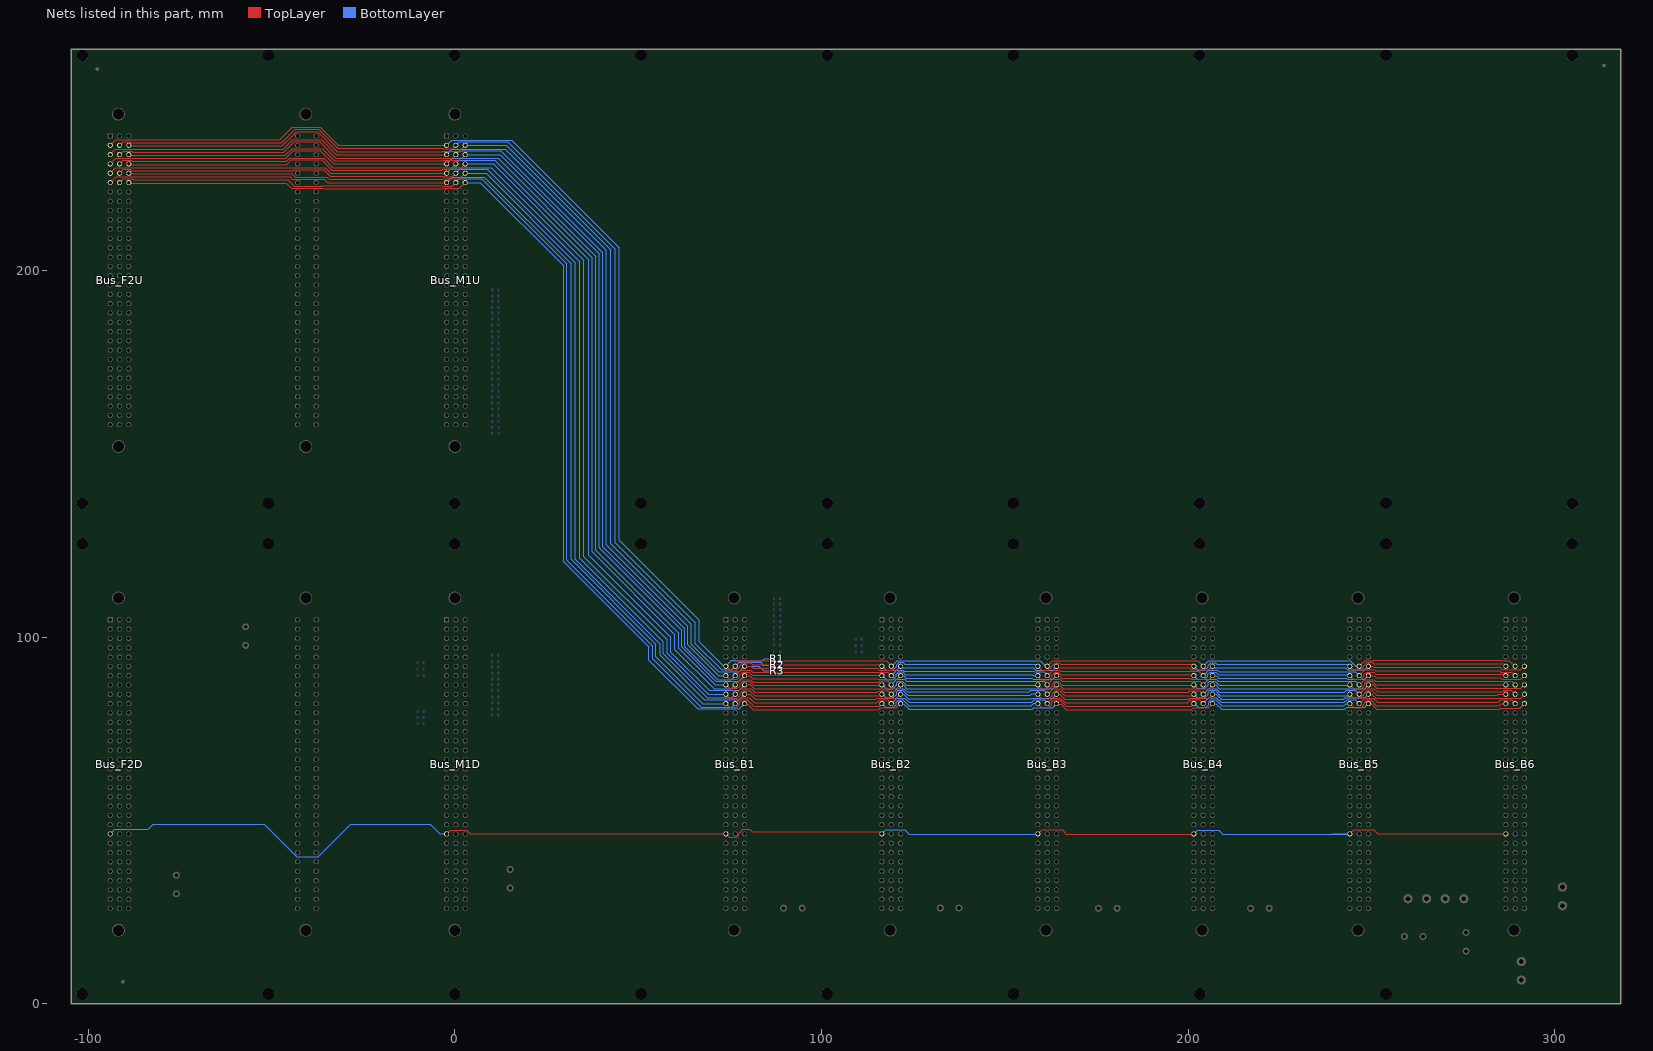
[diagram p0: the nets of this part, all layers, seen from the top]
# Altium PCB MISC67337.PcbDoc (part 4 of 7)
Units mm, origin at the board's own origin, x right, y up, seen from the top; angles counter-clockwise.
Board outline 422.71 x 260.35 mm, 4 copper layers (TopLayer, InternalPlane1, InternalPlane2, BottomLayer); 82 components, 143 nets, 1295 pads, 42 vias.

## Via types
v1: diameter 0.61, hole 0.305, TopLayer to BottomLayer, 42 vias

## Nets (pads, with @x,y where several pads share a name; then routed paths per layer and width w, separated by ;. In a path a pad name is that pad's centre, name@x,y a point inside that pad or via, vN(x,y) a via of type N, cw(c..) or ccw(c..) an arc to the next point about the centre after c; other vN are vias at no path point) (continued)
B_DSP1_XD15: Bus_B1.A24 Bus_B2.A24 Bus_B3.A24 Bus_B4.A24 Bus_B5.A24 Bus_B6.A24 Bus_F2D.A24 Bus_M1D.A24 | length 404.9
  TopLayer w0.254: Bus_M1D.A24@-2.24,46.274 -1.262,47.252 3.245,47.252 4.204,46.293 Bus_B1.A24@73.955,46.293 74.933,45.315 76.9,45.315 77.473,45.888 77.473,46.358 78.613,47.498 80.493,47.498 81.102,46.888 115.91,46.888 Bus_B2.A24@116.505,46.293 ; Bus_B3.A24@159.05,46.166 160.255,47.371 165.633,47.371 166.839,46.165 Bus_B4.A24@201.406,46.165 ; Bus_B4.A24@201.406,46.355 Bus_B4.A24@201.595,46.166 ; Bus_B5.A24@244.14,46.293 245.218,47.371 250.723,47.371 251.801,46.293 Bus_B6.A24@286.685,46.293
  BottomLayer w0.254: Bus_F2D.A24@-93.97,46.274 -92.72,47.523 -83.566,47.523 -82.22,48.87 -52.019,48.87 -43.155,40.005 -37.262,40.005 -28.346,48.92 -6.706,48.92 -4.059,46.274 Bus_M1D.A24@-2.24,46.274 ; Bus_B2.A24@116.505,46.293 117.583,47.371 122.784,47.371 123.896,46.259 151.867,46.259 ; 153.389,46.259 151.867,46.259 ; Bus_B3.A24@159.05,46.293 159.016,46.259 151.867,46.259 ; Bus_B4.A24@201.595,46.293 202.622,47.32 208.407,47.32 209.501,46.227 236.652,46.227 ; 238.352,46.227 236.652,46.227 ; 239.349,46.274 Bus_B5.A24@244.121,46.274 ; Bus_B5.A24@244.14,46.293 Bus_B5.A24@244.121,46.274 ; 236.652,46.227 244.074,46.227 Bus_B5.A24@244.121,46.274
B_DSP2_C\S\: Bus_B1.A6 Bus_B2.A6 Bus_B3.A6 Bus_B4.A6 Bus_B5.A6 Bus_B6.A6 Bus_F2U.A2 Bus_M1U.A2 R1.2 | length 531.8
  TopLayer w0.254: Bus_F2U.A2@-93.97,234.113 -92.473,235.61 -47.701,235.61 -44.298,239.014 -36.728,239.014 -31.828,234.113 Bus_M1U.A2@-2.24,234.113 ; Bus_B1.A6@73.96,92.14 75.295,90.805 76.67,90.805 77.724,91.859 77.724,92.207 78.508,92.991 80.77,92.991 81.31,92.451 109.093,92.451 ; 115.654,92.451 109.093,92.451 ; Bus_B2.A6@116.505,92.013 116.067,92.451 109.093,92.451 ; Bus_B3.A6@159.05,92.013 160.131,90.932 161.925,90.932 162.814,91.821 162.814,92.08 163.725,92.991 164.76,92.991 165.227,92.524 198.374,92.524 ; 200.617,92.524 198.374,92.524 ; Bus_B4.A6@201.595,92.013 201.084,92.524 198.374,92.524 ; Bus_B5.A6@244.14,92.013 245.118,91.035 247.245,91.035 247.904,91.694 247.904,92.08 248.89,93.066 250.19,93.066 250.609,92.646 283.337,92.646 ; 285.707,92.646 283.337,92.646 ; Bus_B6.A6@286.685,92.013 286.052,92.646 283.337,92.646
  BottomLayer w0.254: Bus_M1U.A2@-2.24,234.113 -0.856,235.498 15.505,235.498 44.831,206.172 44.831,126.365 66.675,104.521 66.675,98.679 73.341,92.013 Bus_B1.A6@73.955,92.013 75.538,93.596 76.07,93.596 76.09,93.575 83.796,93.575 84.353,94.132 R1.2@87.097,94.132 ; Bus_B2.A6@116.632,92.075 117.713,90.994 119.507,90.994 120.523,92.01 120.523,92.391 121.185,93.053 122.215,93.053 122.682,92.586 157.505,92.586 ; 158.199,92.586 157.505,92.586 ; Bus_B3.A6@159.05,92.013 158.477,92.586 157.505,92.586 ; Bus_B4.A6@201.595,92.013 202.676,90.932 204.47,90.932 205.486,91.948 205.486,92.329 206.148,92.991 207.411,92.991 207.874,92.528 241.783,92.528 ; 243.162,92.528 241.783,92.528 ; Bus_B5.A6@244.14,92.013 243.625,92.528 241.783,92.528
B_DSP2_X\R\D\: Bus_B1.B6 Bus_B2.B6 Bus_B3.B6 Bus_B4.B6 Bus_B5.B6 Bus_B6.B6 Bus_F2U.B2 Bus_M1U.B2 R2.1 | length 514.3
  TopLayer w0.254: Bus_F2U.B2@-91.43,234.113 -90.452,235.091 -88.485,235.091 -88.161,234.767 -50.317,234.767 ; -49.555,234.767 -50.317,234.767 ; Bus_M1U.B2@0.3,234.113 -0.678,233.136 -3.316,233.136 -3.448,233.267 -31.946,233.267 -37.135,238.455 -43.536,238.455 -47.223,234.767 -50.317,234.767 ; Bus_B1.B6@76.5,92.14 77.908,93.548 117.637,93.548 Bus_B2.B6@119.045,92.14 ; Bus_B3.B6@161.59,92.013 163.049,93.472 202.676,93.472 Bus_B4.B6@204.135,92.013 ; Bus_B5.B6@246.68,92.013 248.242,93.575 250.674,93.575 250.698,93.599 285.496,93.599 285.52,93.575 287.663,93.575 Bus_B6.B6@289.225,92.013
  BottomLayer w0.254: Bus_M1U.B2@0.3,234.113 1.278,235.091 14.489,235.091 43.815,205.765 43.815,125.73 65.659,103.886 65.659,98.171 72.795,91.035 75.517,91.035 Bus_B1.B6@76.495,92.013 77.573,93.091 83.439,93.091 84.201,92.329 87.046,92.329 R2.1@87.097,92.38 ; Bus_B2.B6@119.172,92.075 120.631,93.534 159.704,93.534 161.163,92.075 Bus_B3.B6@161.717,92.075 ; Bus_B4.B6@204.135,92.013 205.594,93.472 244.221,93.472 245.68,92.013 Bus_B5.B6@246.68,92.013
B_DSP2_X\W\E\: Bus_B1.C6 Bus_B2.C6 Bus_B3.C6 Bus_B4.C6 Bus_B5.C6 Bus_B6.C6 Bus_F2U.C2 Bus_M1U.C2 R3.2 | length 513.4
  TopLayer w0.254: Bus_F2U.C2@-88.89,233.924 -47.025,233.924 -43.921,237.028 ; -43.921,237.032 -43.21,237.744 -37.363,237.744 -32.039,232.42 -3.368,232.42 -3.237,232.551 1.278,232.551 Bus_M1U.C2@2.84,234.113 1.391,232.664 ; Bus_B1.C6@79.035,92.013 80.859,92.013 81.367,91.505 112.827,91.505 ; 113.473,91.505 112.827,91.505 ; Bus_B2.C6@121.585,92.14 120.377,90.932 115.849,90.932 115.276,91.505 112.827,91.505 ; Bus_B3.C6@164.13,91.575 198.145,91.575 ; 198.563,91.575 198.145,91.575 ; Bus_B4.C6@206.675,92.013 205.697,91.035 200.887,91.035 200.347,91.575 198.145,91.575 ; Bus_B5.C6@249.22,92.013 249.282,92.075 250.317,92.075 250.698,91.694 283.718,91.694 ; 284.796,91.694 283.718,91.694 ; Bus_B6.C6@291.765,92.013 290.787,91.035 285.774,91.035 285.115,91.694 283.718,91.694
  BottomLayer w0.254: Bus_M1U.C2@2.84,234.113 14.019,234.113 42.545,205.588 42.545,125.476 64.516,103.505 64.516,98.044 72.009,90.551 77.573,90.551 Bus_B1.C6@79.035,92.013 82.969,92.013 84.228,90.754 R3.2@87.097,90.754 ; Bus_B2.C6@121.712,91.638 156.642,91.638 ; 157.353,91.638 156.642,91.638 ; Bus_B3.C6@164.257,92.075 163.114,90.932 158.496,90.932 157.79,91.638 156.642,91.638 ; Bus_B4.C6@206.675,91.584 241.859,91.584 ; 242.632,91.584 241.859,91.584 ; Bus_B5.C6@249.22,92.013 248.242,91.035 243.61,91.035 243.061,91.584 241.859,91.584
B_DSP2_XA0: Bus_B1.A7 Bus_B2.A7 Bus_B3.A7 Bus_B4.A7 Bus_B5.A7 Bus_B6.A7 Bus_F2U.A3 Bus_M1U.A3 | length 507.2
  TopLayer w0.254: Bus_F2U.A3@-93.97,231.573 -93.97,231.658 -92.583,233.045 ; -92.583,233.081 -46.725,233.081 -44.221,235.585 -36.297,235.585 -32.285,231.573 Bus_M1U.A3@-2.24,231.573 ; Bus_B1.A7@73.96,89.473 74.938,88.495 77.065,88.495 77.724,89.154 77.724,89.667 78.508,90.451 80.313,90.451 81.151,89.613 112.141,89.613 ; 112.649,89.613 112.141,89.613 ; Bus_B2.A7@116.505,89.473 116.365,89.613 112.141,89.613 ; Bus_B3.A7@159.05,89.346 160.028,88.368 162.155,88.368 162.814,89.027 162.814,89.54 163.725,90.451 164.667,90.451 165.439,89.679 197.307,89.679 ; 197.739,89.679 197.307,89.679 ; Bus_B4.A7@201.595,89.346 201.468,89.473 Bus_B4.A7@201.595,89.473 201.389,89.679 197.307,89.679 ; Bus_B5.A7@244.14,89.473 245.118,88.495 247.245,88.495 248.031,89.281 248.031,89.789 248.693,90.451 250.671,90.451 251.333,89.789 Bus_B6.A7@286.685,89.789
  BottomLayer w0.254: Bus_M1U.A3@-2.24,231.573 -0.768,233.045 13.716,233.045 41.275,205.486 41.275,125.095 63.5,102.87 63.5,97.917 71.944,89.473 Bus_B1.A7@73.955,89.473 ; Bus_B2.A7@116.632,89.535 117.775,88.392 119.445,88.392 120.396,89.343 120.396,89.851 121.058,90.513 122.136,90.513 122.907,89.742 155.981,89.742 ; 156.818,89.742 155.981,89.742 ; Bus_B3.A7@159.05,89.473 157.858,89.473 157.589,89.742 155.981,89.742 ; Bus_B3.A7@159.05,89.535 Bus_B3.A7@159.177,89.535 ; Bus_B4.A7@201.595,89.473 202.573,88.495 204.573,88.495 205.359,89.281 205.359,89.789 206.021,90.451 207.618,90.451 208.373,89.696 240.462,89.696 ; 241.781,89.696 240.462,89.696 ; Bus_B5.A7@244.14,89.473 243.917,89.696 240.462,89.696
B_DSP2_XA1: Bus_B1.B7 Bus_B2.B7 Bus_B3.B7 Bus_B4.B7 Bus_B5.B7 Bus_B6.B7 Bus_F2U.B3 Bus_M1U.B3 | length 503.5
  TopLayer w0.254: Bus_F2U.B3@-91.43,231.573 -90.452,232.551 -88.121,232.551 -87.808,232.238 -46.603,232.238 -43.764,235.077 -41.758,235.077 ; -41.631,235.077 -41.758,235.077 ; Bus_M1U.B3@0.3,231.573 -0.678,230.596 -32.399,230.596 -36.881,235.077 -41.758,235.077 ; Bus_B1.B7@76.495,89.473 78.006,90.984 80.72,90.984 81.253,90.451 118.067,90.451 Bus_B2.B7@119.045,89.473 ; Bus_B1.B7@76.5,89.473 77.626,90.599 ; Bus_B3.B7@161.59,89.346 163.176,90.932 164.922,90.932 165.227,90.627 202.981,90.627 Bus_B4.B7@204.135,89.473 ; Bus_B4.B7@204.071,89.41 Bus_B4.B7@204.135,89.346 ; Bus_B5.B7@246.68,89.473 248.241,91.034 250.8,91.034 251.092,90.742 285.002,90.742 285.293,90.451 288.247,90.451 Bus_B6.B7@289.225,89.473
  BottomLayer w0.254: Bus_M1U.B3@0.3,231.573 1.365,232.639 12.548,232.639 40.386,204.8 40.386,124.587 62.738,102.235 62.738,97.409 71.755,88.392 75.414,88.392 Bus_B1.B7@76.495,89.473 ; Bus_B2.B7@119.172,89.535 120.62,90.983 122.338,90.983 122.631,90.69 122.682,90.69 157.251,90.69 ; 157.618,90.69 157.251,90.69 ; Bus_B3.B7@161.717,89.535 160.726,90.526 158.075,90.526 157.911,90.69 157.251,90.69 ; Bus_B4.B7@204.135,89.473 205.645,90.983 207.95,90.983 208.458,90.475 245.678,90.475 Bus_B5.B7@246.68,89.473
B_DSP2_XA2: Bus_B1.C7 Bus_B2.C7 Bus_B3.C7 Bus_B4.C7 Bus_B5.C7 Bus_B6.C7 Bus_F2U.C3 Bus_M1U.C3 | length 499.4
  TopLayer w0.254: Bus_F2U.C3@-88.89,231.395 -46.176,231.395 -44.372,233.199 -36.12,233.199 -32.801,229.88 -3.317,229.88 -3.186,230.011 1.278,230.011 Bus_M1U.C3@2.84,231.573 ; Bus_B1.C7@79.035,89.473 80.428,89.473 81.233,88.668 115.372,88.668 115.545,88.495 ; 115.519,88.495 115.545,88.495 ; Bus_B2.C7@121.585,89.473 120.607,88.495 115.545,88.495 ; Bus_B3.C7@164.13,89.473 164.832,89.473 165.575,88.73 197.206,88.73 ; 197.485,88.73 197.206,88.73 ; Bus_B4.C7@206.675,89.346 205.824,88.495 203.73,88.495 203.728,88.494 202.002,88.494 202,88.495 200.863,88.495 200.628,88.73 197.206,88.73 ; Bus_B5.C7@249.22,89.473 250.735,89.473 251.371,88.837 285.356,88.837 285.698,88.495 287.09,88.495 287.114,88.519 288.796,88.519 288.82,88.495 290.787,88.495 Bus_B6.C7@291.765,89.473
  BottomLayer w0.254: Bus_M1U.C3@2.84,231.573 12.343,231.573 39.37,204.546 39.37,124.333 61.849,101.854 61.849,97.282 71.22,87.911 77.473,87.911 Bus_B1.C7@79.035,89.473 ; Bus_B2.C7@121.585,89.473 122.414,89.473 123.093,88.794 156.032,88.794 ; 156.653,88.794 156.032,88.794 ; Bus_B3.C7@164.257,89.535 163.165,88.443 157.745,88.443 157.394,88.794 156.032,88.794 ; Bus_B4.C7@206.675,89.473 207.682,89.473 208.402,88.752 240.665,88.752 ; 241.616,88.752 240.665,88.752 ; Bus_B5.C7@249.22,89.473 248.242,88.495 243.586,88.495 243.329,88.752 240.665,88.752
B_DSP2_XA3: Bus_B1.A8 Bus_B2.A8 Bus_B3.A8 Bus_B4.A8 Bus_B5.A8 Bus_B6.A8 Bus_F2U.A4 Bus_M1U.A4 | length 507.8
  TopLayer w0.254: Bus_F2U.A4@-93.97,229.033 -92.451,230.552 -46.105,230.552 -43.993,232.664 -36.703,232.664 -33.072,229.033 Bus_M1U.A4@-2.24,229.033 ; Bus_B1.A8@73.96,86.933 74.938,85.955 77.065,85.955 77.851,86.741 77.851,87.254 78.508,87.911 80.313,87.911 81.449,86.776 Bus_B2.A8@116.505,86.776 ; Bus_B3.A8@159.05,86.806 160.028,85.828 162.155,85.828 163.093,86.766 163.093,87.279 163.725,87.911 164.667,87.911 165.744,86.834 Bus_B4.A8@201.595,86.834 ; Bus_B5.A8@244.14,86.933 245.221,85.852 247.269,85.852 248.242,86.825 248.242,87.338 248.815,87.911 250.29,87.911 251.269,86.932 286.684,86.932 Bus_B6.A8@286.685,86.933
  BottomLayer w0.254: Bus_M1U.A4@-2.24,229.033 -0.678,230.596 11.797,230.596 38.481,203.911 38.481,123.698 61.087,101.092 61.087,96.901 71.055,86.933 Bus_B1.A8@73.955,86.933 ; Bus_B2.A8@116.632,86.995 117.902,85.725 119.318,85.725 120.523,86.93 120.523,87.565 120.931,87.973 122.034,87.973 123.11,86.898 154.254,86.898 ; 155.929,86.898 154.254,86.898 ; Bus_B3.A8@159.05,86.933 159.015,86.898 154.254,86.898 ; Bus_B4.A8@201.595,86.933 202.573,85.955 204.573,85.955 205.486,86.868 205.486,87.503 205.894,87.911 207.415,87.911 208.461,86.864 238.201,86.864 ; 240.892,86.864 238.201,86.864 ; Bus_B5.A8@244.14,86.933 244.071,86.864 238.201,86.864
B_DSP2_XA4: Bus_B1.B8 Bus_B2.B8 Bus_B3.B8 Bus_B4.B8 Bus_B5.B8 Bus_B6.B8 Bus_F2U.B4 Bus_M1U.B4 | length 500.6
  TopLayer w0.254: Bus_F2U.B4@-91.43,229.033 -90.452,230.011 -88.288,230.011 -87.986,229.709 -45.906,229.709 -44.983,230.632 -35.789,230.632 -33.212,228.056 -0.678,228.056 Bus_M1U.B4@0.3,229.033 ; Bus_B1.B8@76.5,86.933 77.968,88.402 80.559,88.402 81.239,87.722 111.328,87.722 ; 112.258,87.722 111.328,87.722 ; Bus_B2.B8@119.045,86.933 117.94,88.038 115.926,88.038 115.609,87.722 111.328,87.722 ; Bus_B3.B8@161.59,86.806 Bus_B3.B8@161.653,86.87 ; Bus_B3.B8@161.59,86.933 163.074,88.417 165.141,88.417 165.648,87.911 203.157,87.911 Bus_B4.B8@204.135,86.933 ; Bus_B4.B8@204.071,86.87 Bus_B4.B8@204.135,86.806 ; Bus_B5.B8@246.68,86.933 248.139,88.392 250.698,88.392 251.181,87.909 282.473,87.909 282.475,87.911 288.247,87.911 Bus_B6.B8@289.225,86.933
  BottomLayer w0.254: Bus_M1U.B4@0.3,229.033 1.278,230.011 3.245,230.011 3.259,229.997 10.947,229.997 37.465,203.479 37.465,123.19 60.071,100.584 60.071,96.52 70.739,85.852 75.414,85.852 Bus_B1.B8@76.495,86.933 ; Bus_B2.B8@119.045,86.933 120.529,88.417 122.695,88.417 123.139,87.973 160.739,87.973 Bus_B3.B8@161.717,86.995 ; Bus_B4.B8@204.135,86.933 205.619,88.417 207.696,88.417 208.202,87.911 245.702,87.911 Bus_B5.B8@246.68,86.933
B_DSP2_XA5: Bus_B1.C8 Bus_B2.C8 Bus_B3.C8 Bus_B4.C8 Bus_B5.C8 Bus_B6.C8 Bus_F2U.C4 Bus_M1U.C4 | length 501.5
  TopLayer w0.254: Bus_F2U.C4@-88.89,228.866 -45.835,228.866 -44.577,230.124 -36.271,230.124 -33.487,227.34 -3.394,227.34 -3.175,227.559 1.365,227.559 Bus_M1U.C4@2.84,229.033 ; Bus_B1.C8@79.035,86.933 80.529,86.933 81.632,85.83 114.3,85.83 ; 115.189,85.83 114.3,85.83 ; Bus_B2.C8@121.585,86.933 120.482,85.83 114.3,85.83 ; Bus_B3.C8@164.13,86.806 165.035,86.806 165.964,85.877 ; 165.964,85.885 205.746,85.885 ; 205.746,85.877 Bus_B4.C8@206.675,86.806 ; Bus_B5.C8@249.22,86.933 250.455,86.933 251.433,85.955 290.787,85.955 Bus_B6.C8@291.765,86.933
  BottomLayer w0.254: Bus_M1U.C4@2.84,229.033 10.438,229.033 36.576,202.895 36.576,122.301 58.928,99.949 58.928,95.885 69.367,85.446 77.548,85.446 Bus_B1.C8@79.035,86.933 ; Bus_B2.C8@121.585,86.933 122.338,86.933 123.321,85.949 153.924,85.949 ; Bus_B2.C8@121.712,86.995 Bus_B2.C8@122.028,87.311 ; 155.067,85.949 153.924,85.949 ; Bus_B3.C8@164.13,86.933 163.146,85.949 153.924,85.949 ; Bus_B3.C8@164.163,86.901 Bus_B3.C8@164.257,86.995 ; Bus_B4.C8@206.991,87.249 Bus_B4.C8@206.675,86.933 207.529,86.933 208.542,85.921 238.455,85.921 ; 240.03,85.921 238.455,85.921 ; Bus_B5.C8@249.22,86.933 248.208,85.921 238.455,85.921
B_DSP2_XA6: Bus_B1.A9 Bus_B2.A9 Bus_B3.A9 Bus_B4.A9 Bus_B5.A9 Bus_B6.A9 Bus_F2U.A5 Bus_M1U.A5 | length 506
  TopLayer w0.254: Bus_F2U.A5@-93.97,226.493 -92.498,227.965 ; -92.498,228.023 -35.288,228.023 -33.758,226.493 Bus_M1U.A5@-2.24,226.493 ; Bus_B1.A9@73.96,84.393 75.041,83.312 77.089,83.312 77.851,84.074 77.851,84.714 78.532,85.395 78.918,85.395 ; 79.654,85.395 78.918,85.395 ; Bus_B2.A9@116.505,84.393 116.05,83.938 81.899,83.938 80.442,85.395 78.918,85.395 ; Bus_B3.A9@159.05,84.266 160.131,83.185 162.179,83.185 162.941,83.947 162.941,84.587 163.725,85.371 164.997,85.371 166.379,83.988 201.19,83.988 Bus_B4.A9@201.531,84.33 ; Bus_B4.A9@201.152,84.709 Bus_B4.A9@201.531,84.33 ; Bus_B4.A9@201.595,84.266 Bus_B4.A9@201.531,84.33 ; Bus_B4.A9@201.595,84.393 Bus_B4.A9@201.531,84.33 ; Bus_B5.A9@244.14,84.393 245.118,83.415 247.118,83.415 248.242,84.539 248.242,84.798 248.815,85.371 250.239,85.371 251.536,84.074 253.111,84.074 ; 252.73,84.074 253.111,84.074 ; Bus_B6.A9@286.685,84.393 284.621,84.393 284.48,84.252 284.48,84.201 284.353,84.074 253.111,84.074
  BottomLayer w0.254: Bus_M1U.A5@-2.24,226.493 -0.768,227.965 10.008,227.965 35.179,202.794 35.179,121.92 57.912,99.187 57.912,95.631 69.15,84.393 Bus_B1.A9@73.955,84.393 ; Bus_B2.A9@116.632,84.455 117.672,83.415 119.515,83.415 120.523,84.423 120.523,85.025 121.031,85.533 122.137,85.533 123.617,84.053 124.409,84.053 124.435,84.079 ; 124.435,84.053 157.028,84.053 157.429,84.455 Bus_B3.A9@158.988,84.455 ; Bus_B3.A9@159.05,84.393 Bus_B3.A9@158.988,84.455 ; Bus_B3.A9@159.177,84.455 Bus_B3.A9@158.988,84.455 ; Bus_B4.A9@201.595,84.393 202.55,83.438 203.707,83.438 203.73,83.415 204.54,83.415 205.486,84.361 205.486,84.963 205.994,85.471 207.391,85.471 208.829,84.033 238.557,84.033 ; 239.522,84.033 238.557,84.033 ; Bus_B5.A9@244.14,84.393 243.78,84.033 238.557,84.033
B_DSP2_XA7: Bus_B1.B9 Bus_B2.B9 Bus_B3.B9 Bus_B4.B9 Bus_B5.B9 Bus_B6.B9 Bus_F2U.B5 Bus_M1U.B5 | length 508.3
  TopLayer w0.254: Bus_F2U.B5@-91.43,226.493 -90.364,227.559 -88.568,227.559 -88.189,227.18 ; -88.113,227.18 -88.189,227.18 ; Bus_M1U.B5@0.3,226.493 -0.678,225.516 -3.062,225.516 -3.194,225.647 -33.953,225.647 -35.738,227.432 -43.891,227.432 -44.143,227.18 -88.189,227.18 ; Bus_B1.B9@76.5,84.393 78.01,85.903 80.848,85.903 81.867,84.884 115.211,84.884 115.722,85.395 118.043,85.395 Bus_B2.B9@119.045,84.393 ; Bus_B3.B9@161.59,84.266 163.176,85.852 165.353,85.852 166.268,84.937 200.177,84.937 200.611,85.371 203.206,85.371 204.135,84.442 Bus_B4.B9@204.135,84.393 ; Bus_B5.B9@246.68,84.393 248.164,85.877 250.698,85.877 251.549,85.027 253.771,85.027 ; 252.984,85.027 253.771,85.027 ; 284.709,85.027 281.381,85.027 ; Bus_B6.B9@289.225,84.393 288.147,85.471 286.309,85.471 285.865,85.027 281.381,85.027 ; 253.771,85.027 281.381,85.027
  BottomLayer w0.254: Bus_M1U.B5@0.3,226.493 1.365,227.559 8.814,227.559 34.036,202.336 34.036,121.539 56.896,98.679 56.896,95.377 68.858,83.415 75.517,83.415 Bus_B1.B9@76.495,84.393 ; Bus_B2.B9@119.172,84.455 120.656,85.939 122.518,85.939 123.456,85.001 153.67,85.001 ; 155.55,85.001 153.67,85.001 ; Bus_B3.B9@161.717,84.455 160.726,85.446 157.15,85.446 156.706,85.001 153.67,85.001 ; Bus_B4.B9@204.135,84.393 205.619,85.877 207.721,85.877 208.622,84.977 238.785,84.977 ; 240.513,84.977 238.785,84.977 ; Bus_B5.B9@246.68,84.393 245.602,85.471 243.23,85.471 242.736,84.977 238.785,84.977
B_DSP2_XA8: Bus_B1.C9 Bus_B2.C9 Bus_B3.C9 Bus_B4.C9 Bus_B5.C9 Bus_B6.C9 Bus_F2U.C5 Bus_M1U.C5 | length 498.6
  TopLayer w0.254: Bus_F2U.C5@-88.89,226.337 -44.447,226.337 -43.561,225.45 -34.9,225.45 -34.249,224.8 -3.19,224.8 -3.059,224.931 1.278,224.931 Bus_M1U.C5@2.84,226.493 ; Bus_B1.C9@79.035,84.393 80.58,84.393 81.442,83.531 81.446,83.531 81.986,82.992 114.894,82.992 115.24,83.337 116.18,83.337 116.205,83.312 120.377,83.312 Bus_B2.C9@121.585,84.52 ; Bus_B3.C9@164.13,84.393 165.06,84.393 166.413,83.04 200.136,83.04 200.433,83.337 205.619,83.337 Bus_B4.C9@206.675,84.393 ; Bus_B5.C9@249.22,84.393 250.15,84.393 251.231,83.312 290.684,83.312 Bus_B6.C9@291.765,84.393
  BottomLayer w0.254: Bus_M1U.C5@2.84,226.493 8.533,226.493 32.893,202.133 32.893,121.158 56.007,98.044 56.007,94.996 68.072,82.931 77.573,82.931 Bus_B1.C9@79.035,84.393 ; Bus_B2.C9@121.585,84.393 122.439,84.393 123.727,83.105 153.34,83.105 ; 154.494,83.105 153.34,83.105 ; Bus_B3.C9@164.163,84.361 163.114,83.312 157.378,83.312 157.172,83.105 153.34,83.105 ; Bus_B4.C9@206.675,84.393 207.732,84.393 209.037,83.089 238.735,83.089 ; 239.457,83.089 238.735,83.089 ; Bus_B5.C9@249.22,84.393 248.242,83.415 242.799,83.415 242.472,83.089 238.735,83.089
B_DSP2_XA9: Bus_B1.A10 Bus_B2.A10 Bus_B3.A10 Bus_B4.A10 Bus_B5.A10 Bus_B6.A10 Bus_F2U.A6 Bus_M1U.A6 | length 507
  TopLayer w0.254: Bus_F2U.A6@-93.97,223.953 -92.498,225.425 ; -92.498,225.494 -44.874,225.494 -44.272,224.892 -35.56,224.892 -34.622,223.953 Bus_M1U.A6@-2.24,223.953 ; Bus_B1.A10@73.96,81.853 74.938,80.875 76.938,80.875 77.724,81.661 77.724,82.296 78.259,82.831 79.78,82.831 81.511,81.1 115.752,81.1 Bus_B2.A10@116.505,81.853 ; Bus_B3.A10@159.05,81.726 159.901,80.875 162.155,80.875 162.814,81.534 162.814,82.169 163.476,82.831 165.048,82.831 166.735,81.143 200.885,81.143 Bus_B4.A10@201.595,81.853 ; Bus_B5.A10@244.14,81.853 245.221,80.772 247.269,80.772 248.242,81.745 248.242,82.258 248.815,82.831 249.782,82.831 251.396,81.217 284.747,81.217 285.383,81.853 Bus_B6.A10@286.685,81.853 Bus_B6.A10@286.496,82.042
  BottomLayer w0.254: Bus_M1U.A6@-2.24,223.953 -0.768,225.425 8.103,225.425 31.75,201.778 31.75,121.158 54.864,98.044 54.864,94.615 67.626,81.853 Bus_B1.A10@73.955,81.853 ; Bus_B2.A10@116.505,81.853 116.521,81.853 117.499,80.875 119.699,80.875 120.396,81.572 120.396,82.169 121.12,82.893 122.161,82.893 123.845,81.209 152.629,81.209 ; 153.897,81.209 152.629,81.209 ; Bus_B3.A10@159.05,81.853 Bus_B3.A10@158.988,81.915 ; Bus_B3.A10@159.177,81.915 Bus_B3.A10@158.988,81.915 ; Bus_B4.A10@201.595,81.853 201.865,81.853 202.843,80.875 204.954,80.875 205.613,81.534 205.613,82.196 206.248,82.831 207.618,82.831 209.248,81.201 237.668,81.201 ; 238.86,81.201 237.668,81.201 ; Bus_B5.A10@244.14,81.853 243.194,81.853 242.542,81.201 237.668,81.201 ; 152.629,81.209 157.282,81.209 157.988,81.915 Bus_B3.A10@158.988,81.915
B_DSP2_XA10: Bus_B1.B10 Bus_B2.B10 Bus_B3.B10 Bus_B4.B10 Bus_B5.B10 Bus_B6.B10 Bus_F2U.B6 Bus_M1U.B6 | length 510.4
  TopLayer w0.254: Bus_F2U.B6@-91.43,223.953 -90.452,224.931 -87.936,224.931 -87.655,224.651 -47.117,224.651 ; -46.496,224.651 -47.117,224.651 ; Bus_M1U.B6@0.3,223.953 -0.678,222.976 -3.291,222.976 -3.422,223.107 -36.176,223.107 -36.297,222.987 -43.84,222.987 -45.505,224.651 -47.117,224.651 ; Bus_B1.B10@76.5,81.853 78.011,83.364 80.364,83.364 81.682,82.046 85.141,82.046 ; 84.125,82.046 85.141,82.046 ; 114.502,82.046 113.081,82.046 ; Bus_B2.B10@119.045,81.853 117.992,82.906 115.926,82.906 115.066,82.046 113.081,82.046 ; Bus_B3.B10@161.59,81.726 Bus_B3.B10@161.653,81.79 ; Bus_B3.B10@161.59,81.853 163.1,83.363 165.176,83.363 166.447,82.092 199.085,82.092 ; 199.592,82.092 199.085,82.092 ; Bus_B4.B10@204.135,81.853 203.108,82.88 200.736,82.88 199.948,82.092 199.085,82.092 ; Bus_B5.B10@246.68,81.853 248.19,83.363 250.52,83.363 251.713,82.17 254.152,82.17 ; 252.349,82.17 254.152,82.17 ; Bus_B6.B10@289.225,81.853 288.247,82.831 285.244,82.831 284.582,82.17 254.152,82.17 ; 85.141,82.046 113.081,82.046
  BottomLayer w0.254: Bus_M1U.B6@0.3,223.953 1.278,224.931 7.428,224.931 30.607,201.752 30.607,120.904 53.975,97.536 53.975,94.107 67.207,80.875 75.517,80.875 Bus_B1.B10@76.495,81.853 ; Bus_B2.B10@119.172,81.915 120.569,83.312 122.758,83.312 123.913,82.157 152.781,82.157 ; 154.494,82.157 152.781,82.157 ; Bus_B3.B10@161.717,81.915 160.726,82.906 158.064,82.906 157.316,82.157 152.781,82.157 ; Bus_B4.B10@204.135,81.853 205.697,83.415 207.745,83.415 209.015,82.145 237.693,82.145 ; 239.292,82.145 237.693,82.145 ; Bus_B5.B10@246.68,81.853 245.602,82.931 243.459,82.931 242.673,82.145 237.693,82.145
B_DSP2_XA11: Bus_B1.C10 Bus_B2.C10 Bus_B3.C10 Bus_B4.C10 Bus_B5.C10 Bus_B6.C10 Bus_F2U.C6 Bus_M1U.C6 | length 507.4
  TopLayer w0.254: Bus_F2U.C6@-88.89,223.808 -45.906,223.808 -44.526,222.428 -35.956,222.428 -35.789,222.26 -3.404,222.26 -3.272,222.391 1.278,222.391 Bus_M1U.C6@2.84,223.953 ; Bus_B1.C10@79.035,81.853 79.742,81.853 81.441,80.154 113.894,80.154 ; 115.443,80.154 113.894,80.154 ; Bus_B2.C10@121.585,81.853 120.377,80.645 116.103,80.645 115.612,80.154 113.894,80.154 ; Bus_B3.C10@164.13,81.685 165.355,81.685 166.845,80.195 168.605,80.195 ; 167.386,80.195 168.605,80.195 ; 200.533,80.195 197.739,80.195 ; Bus_B4.C10@206.675,81.726 205.721,80.772 201.498,80.772 200.921,80.195 197.739,80.195 ; Bus_B5.C10@249.22,81.853 249.922,81.853 251.51,80.265 252.4,80.265 ; 251.968,80.265 252.4,80.265 ; 290.684,80.772 Bus_B6.C10@291.765,81.853 290.532,80.62 285.217,80.62 284.862,80.265 252.4,80.265 ; 168.605,80.195 197.739,80.195
  BottomLayer w0.254: Bus_M1U.C6@2.84,223.953 6.958,223.953 29.718,201.193 29.718,120.523 52.959,97.282 52.959,93.726 66.267,80.418 77.6,80.418 Bus_B1.C10@79.035,81.853 ; Bus_B2.C10@121.585,81.853 122.363,81.853 123.955,80.261 152.806,80.261 ; 153.732,80.261 152.806,80.261 ; Bus_B3.C10@164.163,81.821 163.114,80.772 157.963,80.772 157.452,80.261 152.806,80.261 ; Bus_B4.C10@206.675,81.853 207.605,81.853 209.201,80.257 237.769,80.257 ; 238.695,80.257 237.769,80.257 ; Bus_B5.C10@249.22,81.853 248.242,80.875 243.434,80.875 242.815,80.257 237.769,80.257